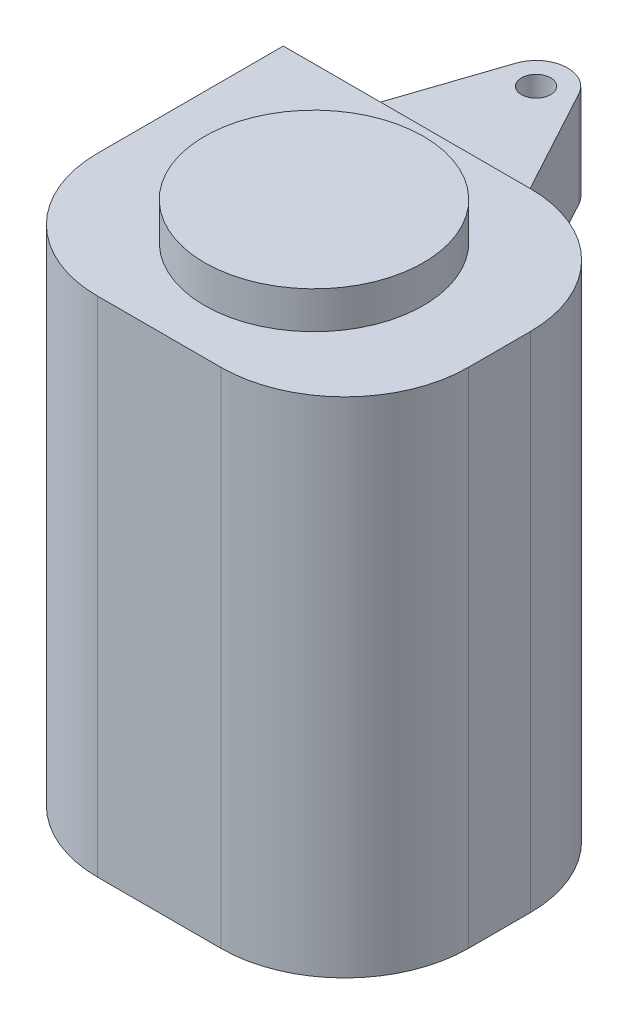
SolidWorks part; units mm, degrees
ref_plane "Front Plane" through (0, 0, 0) normal (0, 0, 1) x (1, 0, 0)
ref_plane "Top Plane" through (0, 0, 0) normal (0, 1, 0) x (1, 0, 0)
ref_plane "Right Plane" through (0, 0, 0) normal (1, 0, 0) x (0, 0, -1)
other "Configuration Table"
sketch "Sketch1" plane through (0, 0, 0) normal (0, 0, 1) x (1, 0, 0)
  line L1 (-39.9868, 20.3289) -> (-10.0306, 20.3289)
  line L2 (-39.9868, 20.3289) -> (-39.9868, -20.3289)
  line L3 (-39.9868, -20.3289) -> (-10.0306, -20.3289)
  line L4 (-10.0306, 20.3289) -> (-10.0306, -20.3289)
  line L5 (-39.9868, 20.3289) -> (-10.0306, -20.3289) construction
  line L6 (-39.9868, -20.3289) -> (-10.0306, 20.3289) construction
  point P0 (-25.0087, 0)
extrude "Boss-Extrude1" add sketch "Sketch1" along normal blind 25
sketch "Sketch2" plane through (0, 0, -4) normal (0, -1, 0) x (1, 0, 0)
  line L0 (-32.2164, -7.0325) -> (-35.914, 4)
  line L1 (-27.5425, -7.4381) -> (-21.3457, 4)
  line L4 (-37.0129, 4) -> (-37.0129, 0)
  line L5 (-37.0129, 0) -> (-13.0045, 0)
  line L6 (-13.0045, 0) -> (-13.0045, 4)
  line L7 (-13.0045, 4) -> (-37.0129, 4)
  line L11 (-21.3457, 4) -> (-35.914, 4)
  arc A0 (-32.2164, -7.0325) -> (-27.5425, -7.4381) centre (-29.7913, -6.2198) ccw
  circle A1 centre (-29.7913, -6.2198) radius 1.1795 construction
  circle A2 centre (-29.7913, -6.2198) radius 1.1795
  dimension "D1" = 0
extrude "Boss-Extrude2" add sketch "Sketch2" along normal mid plane 35
fillet "Fillet1" radius 10 3 edges at (-39.9868, 0, 25) (-10.0306, 0, 0) (-10.0306, 0, 25)
sketch "Sketch3" plane through (0, -20.3289, 0) normal (0, -1, 0) x (-1, 0, 0)
  circle A0 centre (25.0087, -12.5) radius 8.8415
extrude "Boss-Extrude3" add sketch "Sketch3" along normal blind 3
sketch "Sketch4" plane through (0, 20.3289, 0) normal (0, 1, 0) x (1, 0, 0)
  circle A1 centre (-25.0087, -12.5) radius 8.8415
  circle A2 centre (-25.0087, -12.5) radius 8.8415
  dimension "D1" = 0
extrude "Boss-Extrude4" add sketch "Sketch4" along normal blind 3
sketch "Sketch5" plane through (-39.9868, 0, 0) normal (-1, 0, 0) x (0, 0, 1)
  line L0 (-12.7774, 17.5) -> (-12.7774, -17.5) construction
  line L1 (-3.4413, 9.7765) -> (-22.1136, 9.7765)
  line L2 (-3.4413, 9.7765) -> (-3.4413, -9.7765)
  line L3 (-3.4413, -9.7765) -> (-22.1136, -9.7765)
  line L4 (-22.1136, 9.7765) -> (-22.1136, -9.7765)
  line L5 (-3.4413, 9.7765) -> (-22.1136, -9.7765) construction
  line L6 (-3.4413, -9.7765) -> (-22.1136, 9.7765) construction
  point P0 (-12.7774, 0)
extrude "Cut-Extrude1" cut sketch "Sketch5" against normal blind 28
